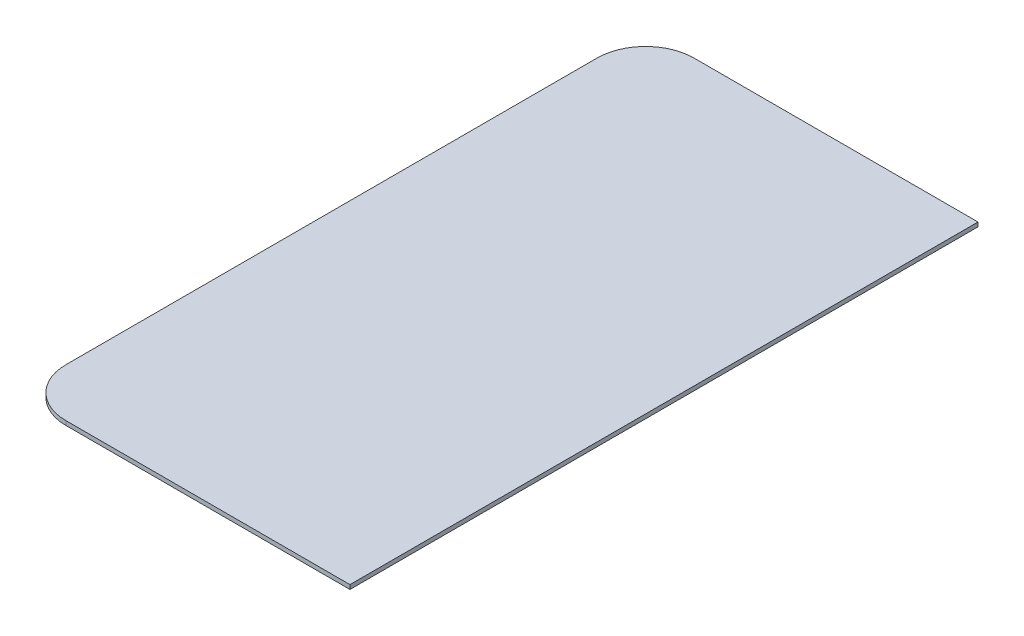
SolidWorks part; units mm, degrees
material "橡木"
ref_plane "Front Plane" through (0, 0, 0) normal (0, 0, 1) x (1, 0, 0)
ref_plane "Top Plane" through (0, 0, 0) normal (0, 1, 0) x (1, 0, 0)
ref_plane "Right Plane" through (0, 0, 0) normal (1, 0, 0) x (0, 0, -1)
sketch "Sketch1" plane through (0, 0, 0) normal (0, 1, 0) x (1, 0, 0)
  line L0 (0, 298) -> (-269.5, 298)
  line L1 (-315.5, 252) -> (-315.5, -252)
  line L2 (-269.5, -298) -> (0, -298)
  line L3 (0, 298) -> (0, -298)
  arc A0 (-269.5, 298) -> (-315.5, 252) centre (-269.5, 252) ccw
  arc A1 (-315.5, -252) -> (-269.5, -298) centre (-269.5, -252) ccw
  dimension "D3" = 46
  dimension "D4" = 46
  dimension "D1" = 596
  dimension "D2" = 315.5
extrude "Boss-Extrude1" add sketch "Sketch1" along normal blind 4
